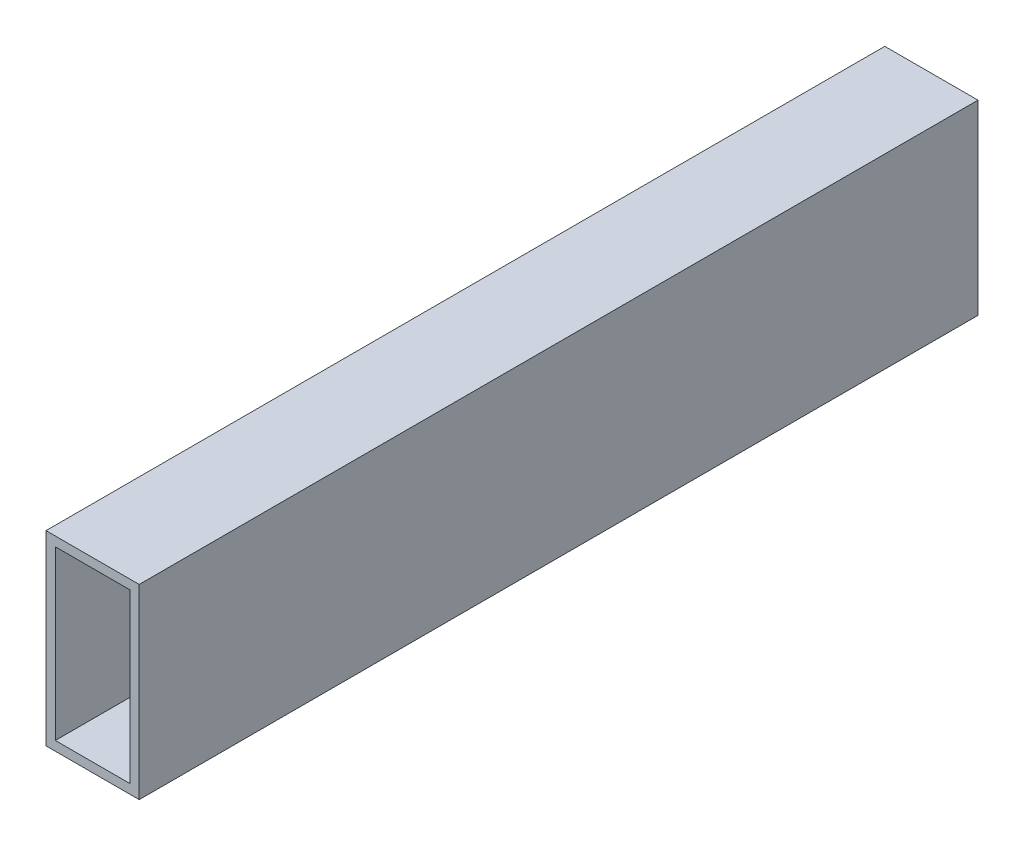
from build123d import *

# Parameters (mm, degrees)
SKETCH_1_W      = 40
SKETCH_1_H      = 80
SKETCH_1_W_2    = 32
SKETCH_1_H_2    = 72
EXTRUDE_1_DEPTH = 180


with BuildPart() as part:
    # 草图1 → 凸台-拉伸1 (new, symmetric)
    with BuildSketch(Plane.XY):
        Rectangle(SKETCH_1_W, SKETCH_1_H)
        Rectangle(SKETCH_1_W_2, SKETCH_1_H_2, mode=Mode.SUBTRACT)
    extrude(amount=EXTRUDE_1_DEPTH, both=True)


solid = part.part
